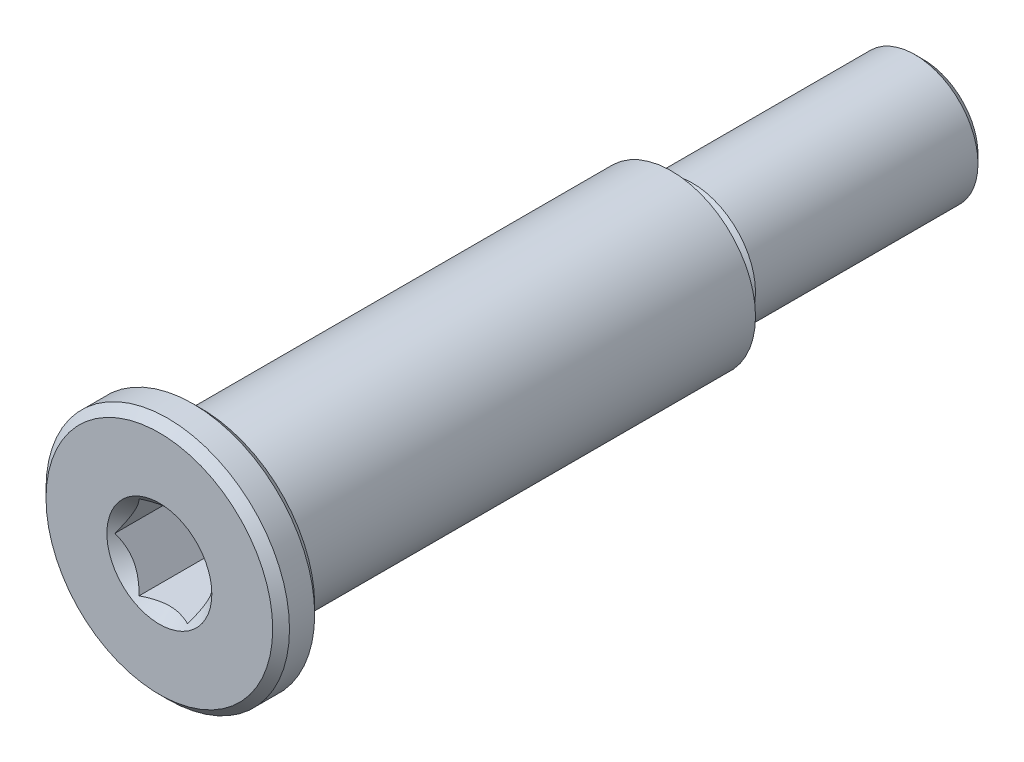
SolidWorks part; units mm, degrees
material "SUS 303"
ref_plane "Front Plane" through (0, 0, 0) normal (0, 0, 1) x (1, 0, 0)
ref_plane "Top Plane" through (0, 0, 0) normal (0, 1, 0) x (1, 0, 0)
ref_plane "Right Plane" through (0, 0, 0) normal (1, 0, 0) x (0, 0, -1)
sketch "Sketch2" plane through (0, 0, 0) normal (0, 1, 0) x (1, 0, 0)
  line L0 (0, 0) -> (2.7, 0)
  line L1 (2.9, 0.2) -> (2.9, 0.8)
  line L2 (2.7, 1) -> (2, 1)
  line L3 (2, 1) -> (2, 12.2)
  line L4 (2, 12.2) -> (1.2, 12.2)
  line L7 (1.5, 12.7) -> (1.5, 18)
  line L8 (1.3, 18.2) -> (0, 18.2)
  line L9 (0, 18.2) -> (0, 0)
  line L10 (0, -4.4259) -> (0, 0) construction
  line L11 (1.5, 12.7) -> (1.2, 12.4)
  line L12 (1.2, 12.4) -> (1.2, 12.2)
  line L13 (1.5, 18) -> (1.3, 18.2)
  line L14 (2.7, 0) -> (2.9, 0.2)
  line L15 (2.9, 0.8) -> (2.7, 1)
  point P1 (2.9, 0)
  point P4 (2.9, 1)
  point P10 (1.5, 18.2)
  dimension "D1" = 4
  dimension "D2" = 3
  dimension "D3" = 5.8
  dimension "D4" = 1
  dimension "D5" = 12.2
  dimension "D6" = 6
  dimension "D7" = 0.5
  dimension "D8" = 0.2
  dimension "D9" = 0.3
revolve "Revolve1" add sketch "Sketch2" angle 360 about L10
cosmetic thread "Cosmetic Thread1" parameters "D2"=2.459
hole_wizard "Size mm Dowel Hole1" positions "Sketch3" profile "Sketch4" hole size "Ø2.0" standard "GB"
sketch "Sketch3" plane through (0, 0, 0) normal (0, 0, 1) x (1, 0, 0)
  point P0 (0, 0)
sketch "Sketch4" plane through (0, 0, 0) normal (1, 0, 0) x (0, -1, 0)
  line L0 (0, 0) -> (0, 3.1009)
  line L1 (0, 3.1009) -> (1, 2.5)
  line L2 (1, 2.5) -> (1, 0.25)
  line L3 (1, 0.25) -> (1.25, 0)
  line L5 (1.25, 0) -> (0, 0)
  line L6 (-1, 0.25) -> (-1.25, 0) construction
  line L10 (0, 3.1009) -> (-1, 2.5) construction
  line L11 (0, -6.35) -> (0, 107.95) construction
  dimension "孔直径" = 2
  dimension "孔深度" = 2.5
  dimension "近端锥形沉头孔直径" = 2.5
  dimension "近端锥形沉头孔角度" = 90
  dimension "导头角度" = 118
sketch "Sketch5" plane through (0, 0, 0) normal (0, 0, 1) x (1, 0, 0)
  line L1 (0.5774, -1) -> (1.1547, 0)
  line L2 (1.1547, 0) -> (0.5774, 1)
  line L3 (0.5774, 1) -> (-0.5774, 1)
  line L4 (-0.5774, 1) -> (-1.1547, 0)
  line L5 (-1.1547, 0) -> (-0.5774, -1)
  line L6 (-0.5774, -1) -> (0.5774, -1)
  circle A0 centre (0, 0) radius 1 construction
  dimension "D1" = 2
extrude "Cut-Extrude1" cut sketch "Sketch5" against normal blind 2.5
